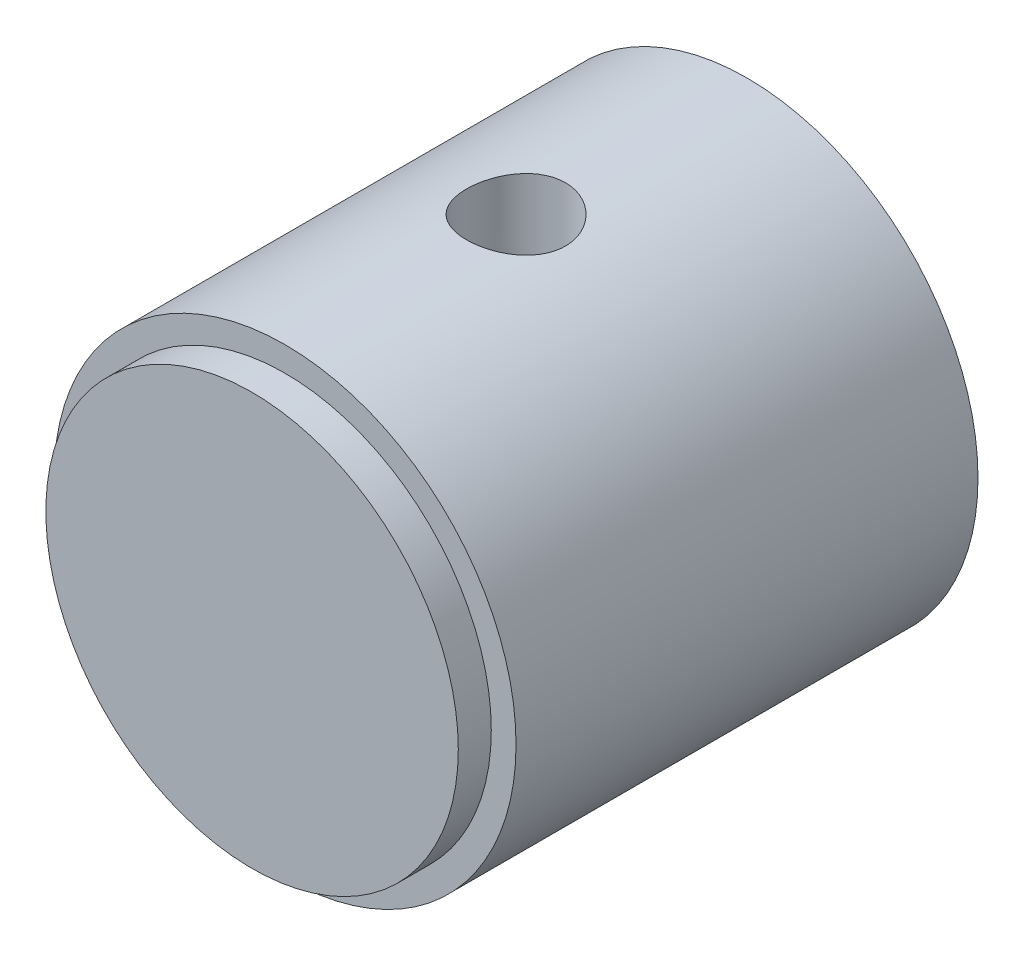
from build123d import *

# Parameters (mm, degrees)
SKETCH1_R                      = 7
BOSS_EXTRUDE1_DEPTH            = 15
CUT_EXTRUDE1_START             = -1
SKETCH2_R                      = 7
SKETCH2_R_2                    = 6.25
CUT_EXTRUDE1_DEPTH             = 1
F_9_5_9_5_DIAMETER_HOLE1_D     = 9.5
F_9_5_9_5_DIAMETER_HOLE1_DEPTH = 11
F_9_5_9_5_DIAMETER_HOLE1_TIP   = 2.85408794
SKETCH4_R                      = 6.2
CUT_EXTRUDE2_DEPTH             = 5
CUT_EXTRUDE2_DRAFT             = -20
SKETCH5_R                      = 1.5
CUT_EXTRUDE3_DEPTH             = 10


with BuildPart() as part:
    # Sketch1 → Boss-Extrude1 (new body)
    with BuildSketch(Plane.XY):
        Circle(SKETCH1_R)
    extrude(amount=BOSS_EXTRUDE1_DEPTH)

    # Sketch2 → Cut-Extrude1 (cut)
    with BuildSketch(Plane.XY.offset(15).offset(CUT_EXTRUDE1_START)):
        Circle(SKETCH2_R)
        Circle(SKETCH2_R_2, mode=Mode.SUBTRACT)
    extrude(amount=CUT_EXTRUDE1_DEPTH, mode=Mode.SUBTRACT)

    # Ø9.5 (9.5) Diameter Hole1
    with Locations(Plane(origin=(0, 0, 0), x_dir=(-1, 0, 0), z_dir=(0, 0, -1))):
        with Locations((0, 0)):
            Hole(F_9_5_9_5_DIAMETER_HOLE1_D / 2, depth=F_9_5_9_5_DIAMETER_HOLE1_DEPTH)
            with Locations((0, 0, -(F_9_5_9_5_DIAMETER_HOLE1_DEPTH + F_9_5_9_5_DIAMETER_HOLE1_TIP / 2))):  # 118° drill point
                Cone(0, F_9_5_9_5_DIAMETER_HOLE1_D / 2, F_9_5_9_5_DIAMETER_HOLE1_TIP, mode=Mode.SUBTRACT)


with BuildPart() as cut_extrude2_tool:
    # Sketch4 → Cut-Extrude2 (with draft: the straight prism first)
    with BuildSketch(Plane(origin=(0, 0, 0), x_dir=(-1, 0, 0), z_dir=(0, 0, -1))):
        Circle(SKETCH4_R)
    extrude(amount=-CUT_EXTRUDE2_DEPTH)
    # Cut-Extrude2: the draft: its side faces are tilted about the plane it starts from
    cut_extrude2_sides = [cut_extrude2_tool.faces().sort_by_distance(p)[0] for p in [
        (6.2, 0, 2.5),
    ]]
    draft(cut_extrude2_sides, Plane(origin=(0, 0, 0), x_dir=(-1, 0, 0), z_dir=(0, 0, -1)), CUT_EXTRUDE2_DRAFT)


with BuildPart() as part_1:
    add(part.part)

    # Cut-Extrude2: cut by cut_extrude2_tool
    add(cut_extrude2_tool.part, mode=Mode.SUBTRACT)

    # Sketch5 → Cut-Extrude3 (cut, symmetric)
    with BuildSketch(Plane(origin=(0, 0, 0), x_dir=(1, 0, 0), z_dir=(0, 1, 0))):
        with Locations(Location((0, -7, 0), (0, 0, 270))):
            Circle(SKETCH5_R)
    extrude(amount=CUT_EXTRUDE3_DEPTH, both=True, mode=Mode.SUBTRACT)


solid = part_1.part
